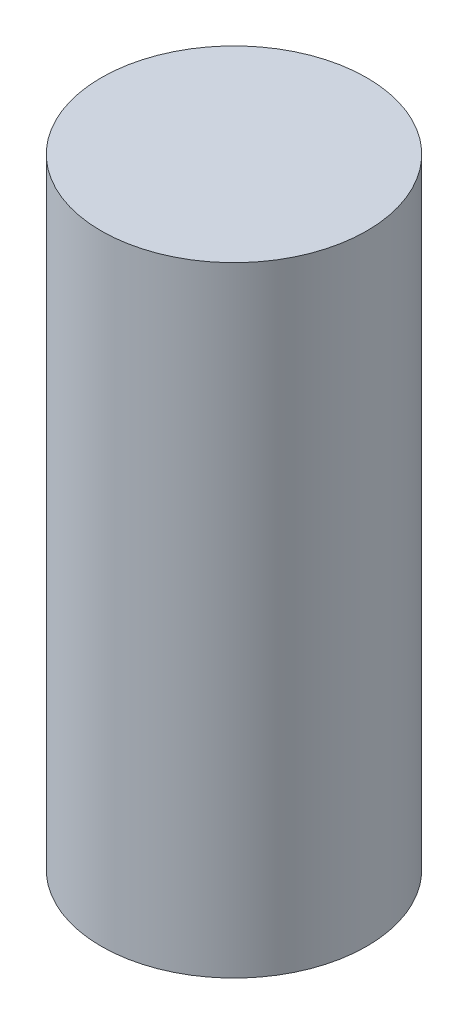
from build123d import *

# Parameters (mm, degrees)
SKETCH1_R              = 15
BOSS_EXTRUDE1_DEPTH    = 35
M20_TAPPED_HOLE1_D     = 17.5
M20_TAPPED_HOLE1_DEPTH = 52.5
M20_TAPPED_HOLE1_TIP   = 5.257530416


with BuildPart() as part:
    # Sketch1 → Boss-Extrude1 (new, symmetric)
    with BuildSketch(Plane(origin=(0, 0, 0), x_dir=(1, 0, 0), z_dir=(0, 1, 0))):
        with Locations(Location((0, 0, 0), (0, 0, 270))):
            Circle(SKETCH1_R)
    extrude(amount=BOSS_EXTRUDE1_DEPTH, both=True)

    # M20 Tapped Hole1
    with Locations(Plane(origin=(0, -35, 0), x_dir=(0, 0, -1), z_dir=(0, -1, 0))):
        with Locations((0, 0)):
            Hole(M20_TAPPED_HOLE1_D / 2, depth=M20_TAPPED_HOLE1_DEPTH)
            with Locations((0, 0, -(M20_TAPPED_HOLE1_DEPTH + M20_TAPPED_HOLE1_TIP / 2))):  # 118° drill point
                Cone(0, M20_TAPPED_HOLE1_D / 2, M20_TAPPED_HOLE1_TIP, mode=Mode.SUBTRACT)


solid = part.part
